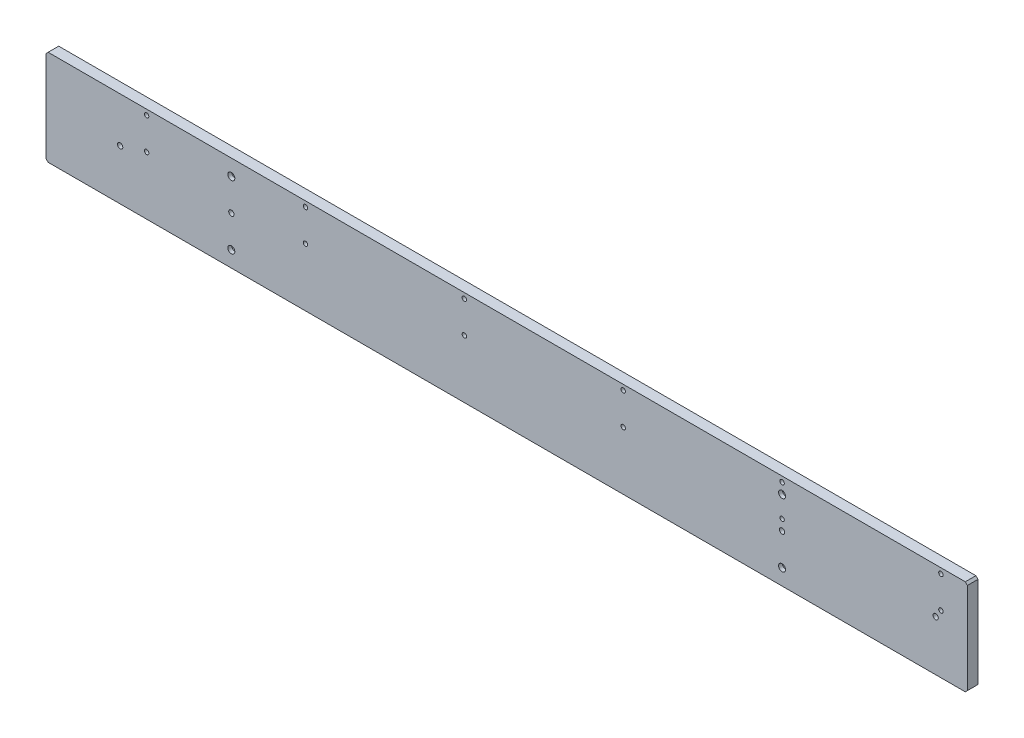
SolidWorks part; units mm, degrees
material "45号钢"
ref_plane "主视基准图" through (0, 0, 0) normal (0, 0, 1) x (1, 0, 0)
ref_plane "上视基准图" through (0, 0, 0) normal (0, 1, 0) x (1, 0, 0)
ref_plane "右视基准图" through (0, 0, 0) normal (1, 0, 0) x (0, 0, -1)
sketch "草图1" plane through (0, 0, 0) normal (0, 0, 1) x (1, 0, 0)
  line L1 (-435, -45) -> (435, -45)
  line L2 (-435, -45) -> (-435, 45)
  line L3 (-435, 45) -> (435, 45)
  line L4 (435, -45) -> (435, 45)
  line L5 (-435, -45) -> (435, 45) construction
  line L6 (-435, 45) -> (435, -45) construction
  point P0 (0, 0)
  dimension "D1" = 870
  dimension "D2" = 90
extrude "凸台-拉伸1" add sketch "草图1" along normal blind 10
chamfer "倒角1" distance 2 angle 45 4 edges at (435, 45, 5) (435, -45, 5) (-435, 45, 5) (-435, -45, 5)
hole_wizard "M6 六角凹头螺钉的柱形沉头孔1" positions "草图3" profile "草图2" counterbore size "M6" standard "Iso" end condition through all
sketch "草图3" plane through (0, 0, 0) normal (0, 0, -1) x (-1, 0, 0)
  point P0 (-260, 30)
  point P3 (-260, -30)
  point P6 (260, -30)
  point P9 (260, 30)
  point P17 (-105.2444, -69.2506)
  dimension "D1" = 520
  dimension "D2" = 260
sketch "草图2" plane through (260, 30, 0) normal (1, 0, 0) x (0, 1, 0)
  line L0 (0, 0) -> (0, 10)
  line L1 (0, 10) -> (3.3, 10)
  line L3 (3.3, 10) -> (3.3, 6.4)
  line L4 (3.3, 6.4) -> (5.5, 6.4)
  line L5 (5.5, 6.4) -> (5.5, 0)
  line L7 (5.5, 0) -> (0, 0)
  line L11 (0, -6.35) -> (0, 107.95) construction
  dimension "通孔孔直径" = 6.6
  dimension "通孔孔深度" = 10
  dimension "柱形沉头孔直径" = 11
  dimension "柱形沉头孔深度" = 6.4
hole_wizard "Ø5.0 (5) 直径孔1" positions "草图5" profile "草图4" hole size "Ø5.0" standard "Ansi Metric"
sketch "草图5" plane through (0, 0, 0) normal (0, 0, -1) x (-1, 0, 0)
  point P0 (-260, 0)
  point P3 (260, 0)
sketch "草图4" plane through (260, 0, 0) normal (1, 0, 0) x (0, 1, 0)
  line L0 (0, 0) -> (0, 17.0534)
  line L1 (0, 17.0534) -> (2.5, 15.61)
  line L2 (2.5, 15.61) -> (2.5, 0)
  line L5 (2.5, 0) -> (0, 0)
  line L10 (0, 17.0534) -> (-2.5, 15.61) construction
  line L11 (0, -6.35) -> (0, 107.95) construction
  dimension "孔直径" = 5
  dimension "孔深度" = 15.61
  dimension "导头角度" = 120
sketch "草图8" plane through (0, 0, 0) normal (0, 0, -1) x (-1, 0, 0)
  line L0 (433, -45) -> (-433, -45) construction
  line L1 (-435, -43) -> (-435, 43) construction
  circle A0 centre (365, 2.5) radius 2.5
  circle A2 centre (-405, 2.5) radius 2.5
  dimension "D1" = 47.5
  dimension "D2" = 30
  dimension "D5" = 5
extrude "切除-拉伸1" cut sketch "草图8" against normal through all
hole_wizard "M5 螺纹孔2" positions "草图10" profile "草图9" tap size "M5" standard "Iso"
sketch "草图10" plane through (0, 0, 10) normal (0, 0, 1) x (1, 0, 0)
  line L1 (435, -43) -> (435, 43) construction
  line L3 (433, 45) -> (-433, 45) construction
  point P0 (410, 40)
  point P2 (410, 10)
  dimension "D1" = 30
  dimension "D2" = 25
  dimension "D3" = 5
sketch "草图9" plane through (410, 40, 10) normal (1, 0, 0) x (0, -1, 0)
  line L0 (0, 0) -> (0, 18.6618)
  line L1 (0, 18.6618) -> (2.1, 17.4)
  line L2 (2.1, 17.4) -> (2.1, 0)
  line L5 (2.1, 0) -> (0, 0)
  line L10 (0, 18.6618) -> (-2.1, 17.4) construction
  line L11 (0, -6.35) -> (0, 107.95) construction
  dimension "螺纹孔钻头直径" = 4.2
  dimension "螺纹孔钻头深度" = 17.4
  dimension "导头角度" = 118
cosmetic thread "孔螺蚊线5" parameters "D1"=10, "D2"=5
cosmetic thread "孔螺蚊线6" parameters "D1"=10, "D2"=5
pattern_linear "阵列(线性)1" count 6 spacing 150 along (-1, 0, 0) of "M5 螺纹孔2"
hole_wizard "M3 螺纹孔1" positions "草图12" profile "草图11" tap size "M3" standard "Iso"
sketch "草图12" plane through (0, 0, 0) normal (0, 0, -1) x (-1, 0, 0)
  line L0 (435, 43) -> (435, -43) construction
  point P0 (317, -16.4)
  point P2 (317, -40)
  point P4 (335, -40)
  point P6 (335, -16.4)
  dimension "D1" = 18
  dimension "D2" = 23.6
  dimension "D3" = 100
sketch "草图11" plane through (-317, -16.4, 0) normal (1, 0, 0) x (0, 1, 0)
  line L0 (0, 0) -> (0, 8.2511)
  line L1 (0, 8.2511) -> (1.25, 7.5)
  line L2 (1.25, 7.5) -> (1.25, 0)
  line L5 (1.25, 0) -> (0, 0)
  line L10 (0, 8.2511) -> (-1.25, 7.5) construction
  line L11 (0, -6.35) -> (0, 107.95) construction
  dimension "螺纹孔钻头直径" = 2.5
  dimension "螺纹孔钻头深度" = 7.5
  dimension "导头角度" = 118
cosmetic thread "孔螺蚊线7" parameters "D1"=6, "D2"=3
cosmetic thread "孔螺蚊线8" parameters "D1"=6, "D2"=3
cosmetic thread "孔螺蚊线9" parameters "D1"=6, "D2"=3
cosmetic thread "孔螺蚊线10" parameters "D1"=6, "D2"=3
